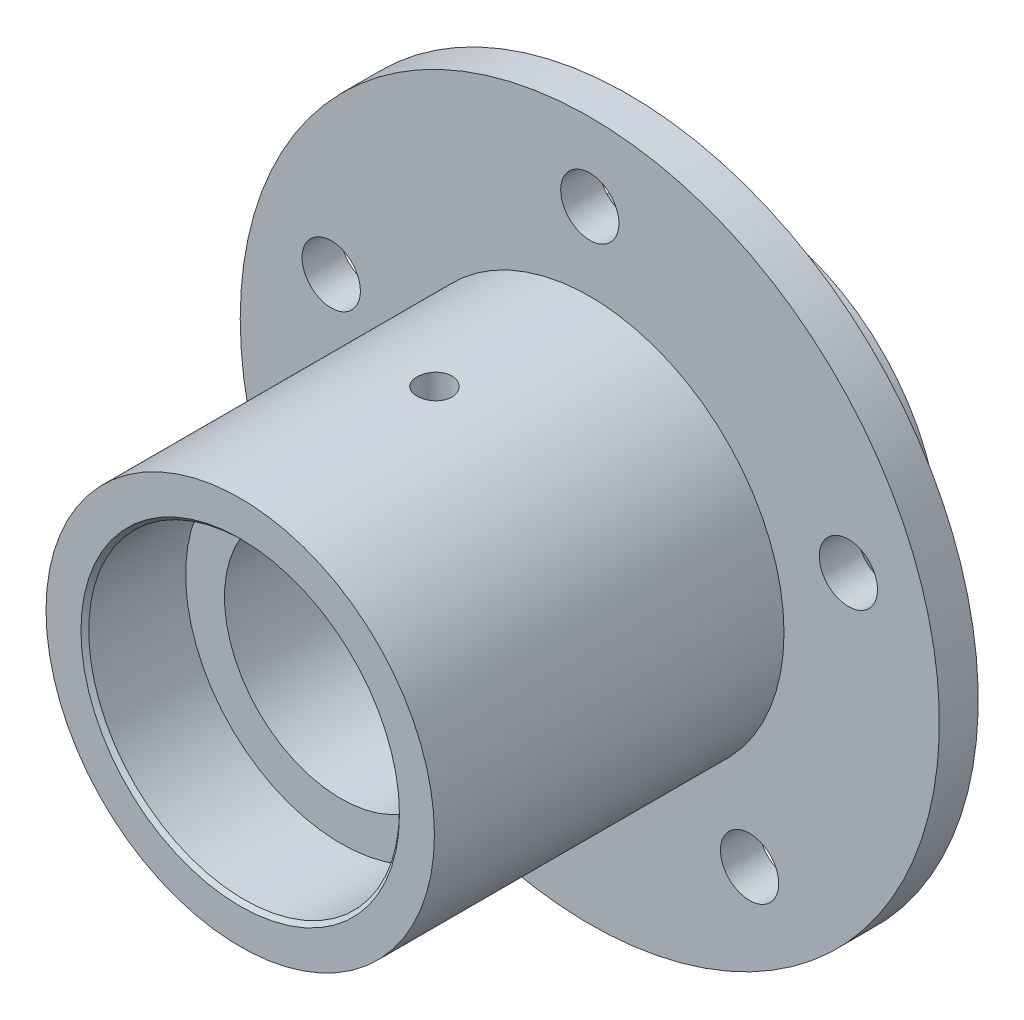
from build123d import *

# Parameters (mm, degrees)
EXTRUDE_1_DEPTH             = 120
EXTRUDE_1_DEPTH_BACK        = 10
SKETCH_1_R                  = 50
SKETCH_2_R                  = 30
CUT_EXTRUDE_1_DEPTH         = 120
SKETCH_3_R                  = 40
CUT_EXTRUDE_2_DEPTH         = 25.95
CUT_EXTRUDE_START           = -35.95
SKETCH_4_R                  = 40
CUT_EXTRUDE_3_DEPTH         = 35.95
SKETCH_6_R                  = 90
SKETCH_6_R_2                = 50
EXTRUDE_2_DEPTH             = 10
SKETCH_7_R                  = 2.5
CUT_EXTRUDE_5_DEPTH         = 30
SKETCH_11_R                 = 7.5
CUT_EXTRUDE_6_DEPTH         = 10
CUT_EXTRUDE_START_2         = -2.7
SKETCH_12_R                 = 41.75
SKETCH_12_R_2               = 40
CUT_EXTRUDE_7_DEPTH         = 2.7
HOLE_WIZARD_M6_1_AT_2_COUNT = 2
HOLE_WIZARD_M6_1_AT_2_PITCH = 45
HOLE_WIZARD_M6_1_AT_3_COUNT = 2
HOLE_WIZARD_M6_1_AT_3_PITCH = 77.942286341
HOLE_WIZARD_M6_1_AT_4_COUNT = 2
HOLE_WIZARD_M6_1_AT_4_PITCH = 90
HOLE_WIZARD_M6_1_AT_5_COUNT = 2
HOLE_WIZARD_M6_1_AT_5_PITCH = 77.942286341
HOLE_WIZARD_M6_1_AT_6_COUNT = 2
HOLE_WIZARD_M6_1_AT_6_PITCH = 45
CHAMFER_1_SIZE              = 1


with BuildPart() as part:
    # 草图1 → 凸台-拉伸1 (new, two sides: drawn at the far end of the back side and taken through both)
    with BuildSketch(Plane.XY.offset(-EXTRUDE_1_DEPTH_BACK)):
        Circle(SKETCH_1_R)
    extrude(amount=EXTRUDE_1_DEPTH + EXTRUDE_1_DEPTH_BACK)

    # 草图2 → 切除-拉伸1 (cut)
    with BuildSketch(Plane.XY.offset(120)):
        Circle(SKETCH_2_R)
    extrude(amount=-CUT_EXTRUDE_1_DEPTH, mode=Mode.SUBTRACT)

    # 草图3 → 切除-拉伸2 (cut)
    with BuildSketch(Plane.XY.offset(120)):
        Circle(SKETCH_3_R)
    extrude(amount=-CUT_EXTRUDE_2_DEPTH, mode=Mode.SUBTRACT)

    # 草图4 → 切除-拉伸3 (cut)
    with BuildSketch(Plane(origin=(0, 0, -10), x_dir=(-1, 0, 0), z_dir=(0, 0, -1)).offset(CUT_EXTRUDE_START)):
        with Locations(Location((0, 0, 0), (0, 0, 180))):
            Circle(SKETCH_4_R)
    extrude(amount=CUT_EXTRUDE_3_DEPTH, mode=Mode.SUBTRACT)

    # 草图7 → 切除-拉伸5 (cut)
    with BuildSketch(Plane(origin=(0, 50, 0), x_dir=(1, 0, 0), z_dir=(0, 1, 0))):
        with Locations(Location((0, -70, 0), (0, 0, 270))):
            Circle(SKETCH_7_R)
    extrude(amount=-CUT_EXTRUDE_5_DEPTH, mode=Mode.SUBTRACT)

    # 草图8 → M10x1.0 螺纹孔1 (revolve, cut)
    with BuildSketch(Plane(origin=(0, 50, 70), x_dir=(0, 0, 1), z_dir=(1, 0, 0))):
        Polygon((0, 0), (0, 11), (4.5, 8.296127214), (4.5, 0), align=None)
    revolve(axis=Axis((0, 56.35, 70), (0, -1, 0)), mode=Mode.SUBTRACT)

    # 草图12 → 切除-拉伸7 (cut)
    with BuildSketch(Plane(origin=(0, 0, 5.3), x_dir=(-1, 0, 0), z_dir=(0, 0, -1)).offset(CUT_EXTRUDE_START_2)):
        Circle(SKETCH_12_R)
        Circle(SKETCH_12_R_2, mode=Mode.SUBTRACT)
    extrude(amount=CUT_EXTRUDE_7_DEPTH, mode=Mode.SUBTRACT)

    # 草图17 → M6 螺纹孔1 (revolve, cut)
    with BuildSketch(Plane(origin=(0, 45, -10), x_dir=(0, 1, 0), z_dir=(1, 0, 0))):
        Polygon((0, 0), (0, 16.502151548), (2.5, 15), (2.5, 0), align=None)
    hole_wizard_m6_1 = revolve(axis=Axis((0, 45, -16.35), (0, 0, 1)), mode=Mode.SUBTRACT)

    # M6 螺纹孔1 at 2: M6 螺纹孔1 ×2
    with Locations(*[Vector(-0.8660254037844528, -0.4999999999999755, 0) * (i * HOLE_WIZARD_M6_1_AT_2_PITCH) for i in range(1, HOLE_WIZARD_M6_1_AT_2_COUNT)]):
        add(hole_wizard_m6_1, mode=Mode.SUBTRACT)

    # M6 螺纹孔1 at 3: M6 螺纹孔1 ×2
    with Locations(*[Vector(-0.5000000000000245, -0.8660254037844246, 0) * (i * HOLE_WIZARD_M6_1_AT_3_PITCH) for i in range(1, HOLE_WIZARD_M6_1_AT_3_COUNT)]):
        add(hole_wizard_m6_1, mode=Mode.SUBTRACT)

    # M6 螺纹孔1 at 4: M6 螺纹孔1 ×2
    with Locations(*[(0, -i * HOLE_WIZARD_M6_1_AT_4_PITCH, 0) for i in range(1, HOLE_WIZARD_M6_1_AT_4_COUNT)]):
        add(hole_wizard_m6_1, mode=Mode.SUBTRACT)

    # M6 螺纹孔1 at 5: M6 螺纹孔1 ×2
    with Locations(*[Vector(0.4999999999999754, -0.8660254037844529, 0) * (i * HOLE_WIZARD_M6_1_AT_5_PITCH) for i in range(1, HOLE_WIZARD_M6_1_AT_5_COUNT)]):
        add(hole_wizard_m6_1, mode=Mode.SUBTRACT)

    # M6 螺纹孔1 at 6: M6 螺纹孔1 ×2
    with Locations(*[Vector(0.8660254037844243, -0.500000000000025, 0) * (i * HOLE_WIZARD_M6_1_AT_6_PITCH) for i in range(1, HOLE_WIZARD_M6_1_AT_6_COUNT)]):
        add(hole_wizard_m6_1, mode=Mode.SUBTRACT)

    # 倒角1
    chamfer_1_edges = [part.edges().sort_by_distance(p)[0] for p in [
        (-40, 0, 120),
        (-40, 0, -10),
    ]]
    chamfer(chamfer_1_edges, length=CHAMFER_1_SIZE)


with BuildPart() as body_2:
    # 草图6 → 凸台-拉伸2 (new body)
    with BuildSketch(Plane(origin=(0, 0, 20), x_dir=(-1, 0, 0), z_dir=(0, 0, -1))):
        Circle(SKETCH_6_R)
        Circle(SKETCH_6_R_2, mode=Mode.SUBTRACT)
    extrude(amount=-EXTRUDE_2_DEPTH)

    # 草图11 → 切除-拉伸6 (cut)
    with BuildSketch(Plane(origin=(0, 0, 20), x_dir=(-1, 0, 0), z_dir=(0, 0, -1))):
        with Locations((0, 70)):
            Circle(SKETCH_11_R)
        with Locations((66.573956141, 21.631189606)):
            Circle(SKETCH_11_R)
        with Locations((41.14496766, -56.631189606)):
            Circle(SKETCH_11_R)
        with Locations((-41.14496766, -56.631189606)):
            Circle(SKETCH_11_R)
        with Locations((-66.573956141, 21.631189606)):
            Circle(SKETCH_11_R)
    extrude(amount=-CUT_EXTRUDE_6_DEPTH, mode=Mode.SUBTRACT)


solid = Compound([part.part, body_2.part])
